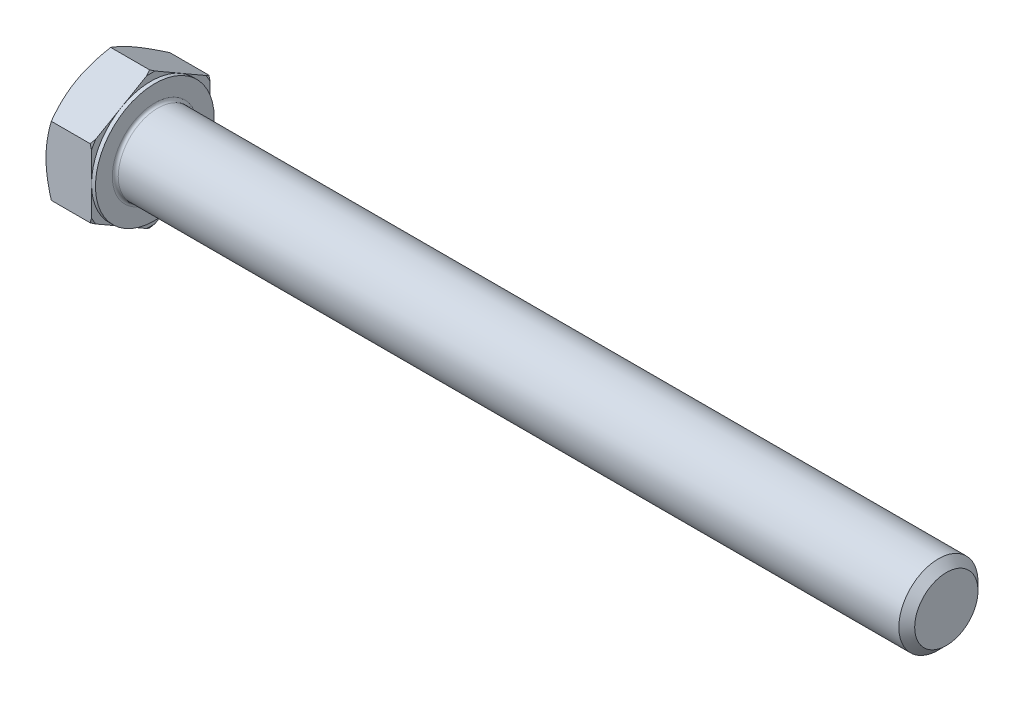
from build123d import *

# Parameters (mm, degrees)
BASE_EXTRUDE_DEPTH = 10
SKETCH4_W          = 0.8
SKETCH4_H          = 11.856406461
CHAMFER_2_SIZE     = 1.6
FILLET_2_R         = 0.6


with BuildPart() as part:
    # Sketch1 → Base-Extrude (new body)
    with BuildSketch(Plane(origin=(0, 0, 0), x_dir=(0, 0, -1), z_dir=(1, 0, 0))):
        Polygon((12, 6.92820323), (12, -6.92820323), (0, -13.856406461), (-12, -6.92820323), (-12, 6.92820323), (0, 13.856406461), align=None)
    extrude(amount=BASE_EXTRUDE_DEPTH)

    # Sketch2 → Boss-Revolve1 (revolve)
    with BuildSketch(Plane.XY, mode=Mode.PRIVATE) as boss_revolve1_sk:
        Polygon((0, 0), (170, 0), (170, 6.268), (170, 8), (0, 8), align=None)
    revolve(boss_revolve1_sk.sketch.rotate(Axis((0, 0, 0), (1, 0, 0)), 90), axis=Axis((0, 0, 0), (1, 0, 0)))

    # Sketch3 → Cut-Revolve1 (revolve, cut)
    with BuildSketch(Plane.XY):
        Polygon((0, 12), (3.958548116, 18.856406461), (3.958548116, 23.856406461), (-10, 23.856406461), (-10, 12), align=None)
    revolve(axis=Axis((0, 0, 0), (1, 0, 0)), mode=Mode.SUBTRACT)

    # Sketch5 → Cut-Revolve2 (revolve, cut)
    with BuildSketch(Plane.XY):
        Polygon((10, 12), (6.041451884, 18.856406461), (6.041451884, 23.856406461), (16.041451884, 23.856406461), (16.041451884, 12), align=None)
    revolve(axis=Axis((0, 0, 0), (1, 0, 0)), mode=Mode.SUBTRACT)

    # Sketch4 → Cut-Revolve3 (revolve, cut)
    with BuildSketch(Plane.XY, mode=Mode.PRIVATE) as cut_revolve3_sk:
        with Locations((9.6, 17.928203231)):
            Rectangle(SKETCH4_W, SKETCH4_H)
    revolve(cut_revolve3_sk.sketch.rotate(Axis((0, 0, 0), (1, 0, 0)), 270), axis=Axis((0, 0, 0), (1, 0, 0)), mode=Mode.SUBTRACT)

    # Chamfer 2
    chamfer_2_edges = [part.edges().sort_by_distance(p)[0] for p in [
        (170, 0, -8),
    ]]
    chamfer(chamfer_2_edges, length=CHAMFER_2_SIZE)

    # Fillet 2
    fillet_2_edges = [part.edges().sort_by_distance(p)[0] for p in [
        (10, 0, -8),
    ]]
    fillet(fillet_2_edges, radius=FILLET_2_R)


solid = part.part
